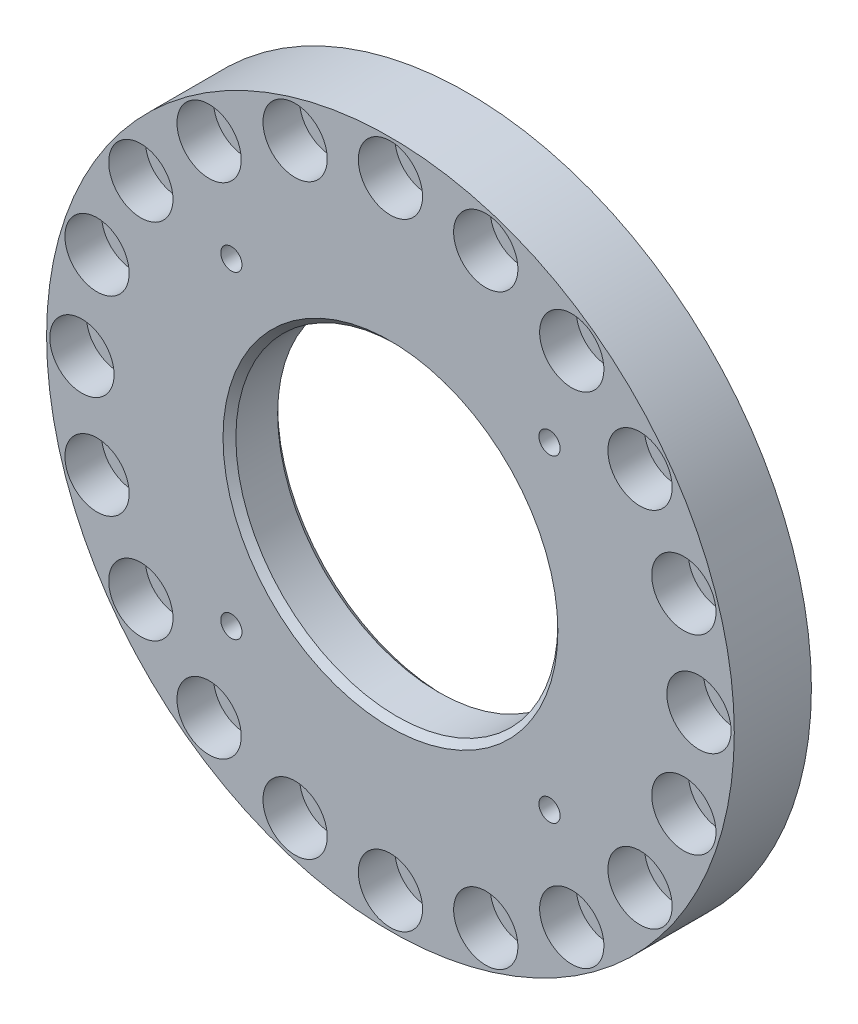
from build123d import *

# Parameters (mm, degrees)
SKETCH_1_R                = 53.5
SKETCH_1_R_2              = 25.05
EXTRUDE_1_DEPTH           = 6
HOLE_WIZARD_1_D           = 5.5
HOLE_WIZARD_1_CBORE_D     = 10
HOLE_WIZARD_1_CBORE_DEPTH = 5.7
SKETCH_6_R                = 33.55
CUT_EXTRUDE_1_DEPTH       = 3.5
CHAMFER_1_SIZE            = 1
HOLE_WIZARD_M4_1_D        = 3.3
PATTERN_CIRCULAR_1_COUNT  = 20
PATTERN_CIRCULAR_2_COUNT  = 4


with BuildPart() as part:
    # 草图1 → 凸台-拉伸1 (new, symmetric)
    with BuildSketch(Plane.XY):
        Circle(SKETCH_1_R)
        Circle(SKETCH_1_R_2, mode=Mode.SUBTRACT)
    extrude(amount=EXTRUDE_1_DEPTH, both=True)

    # 打孔尺寸(%根据)内六角圆柱头螺钉的类型1 (through all)
    with Locations(Plane.XY.offset(6)):
        with Locations((0, 48)):
            hole_wizard_1 = CounterBoreHole(HOLE_WIZARD_1_D / 2, HOLE_WIZARD_1_CBORE_D / 2, HOLE_WIZARD_1_CBORE_DEPTH)

    # 草图6 → 切除-拉伸1 (cut)
    with BuildSketch(Plane(origin=(0, 0, -6), x_dir=(-1, 0, 0), z_dir=(0, 0, -1))):
        Circle(SKETCH_6_R)
    extrude(amount=-CUT_EXTRUDE_1_DEPTH, mode=Mode.SUBTRACT)

    # 倒角1
    chamfer_1_edges = [part.edges().sort_by_distance(p)[0] for p in [
        (-25.05, 0, -2.5),
        (33.55, 0, -6),
        (-25.05, 0, 6),
    ]]
    chamfer(chamfer_1_edges, length=CHAMFER_1_SIZE)

    # M4 螺纹孔1 (through all)
    with Locations(Plane.XY.offset(6)):
        with Locations((24.748737342, 24.748737342)):
            hole_wizard_m4_1 = Hole(HOLE_WIZARD_M4_1_D / 2)

    # 阵列(圆周)1: 打孔尺寸(%根据)内六角圆柱头螺钉的类型1 ×20 about axis
    pattern_circular_1_axis = Axis((0, 0, 0), (0, 0, 1))
    for i in range(1, PATTERN_CIRCULAR_1_COUNT):
        add(hole_wizard_1.rotate(pattern_circular_1_axis, i * 360 / PATTERN_CIRCULAR_1_COUNT), mode=Mode.SUBTRACT)

    # 阵列(圆周)2: M4 螺纹孔1 ×4 about axis
    pattern_circular_2_axis = Axis((0, 0, 0), (0, 0, 1))
    for i in range(1, PATTERN_CIRCULAR_2_COUNT):
        add(hole_wizard_m4_1.rotate(pattern_circular_2_axis, i * 360 / PATTERN_CIRCULAR_2_COUNT), mode=Mode.SUBTRACT)


solid = part.part
